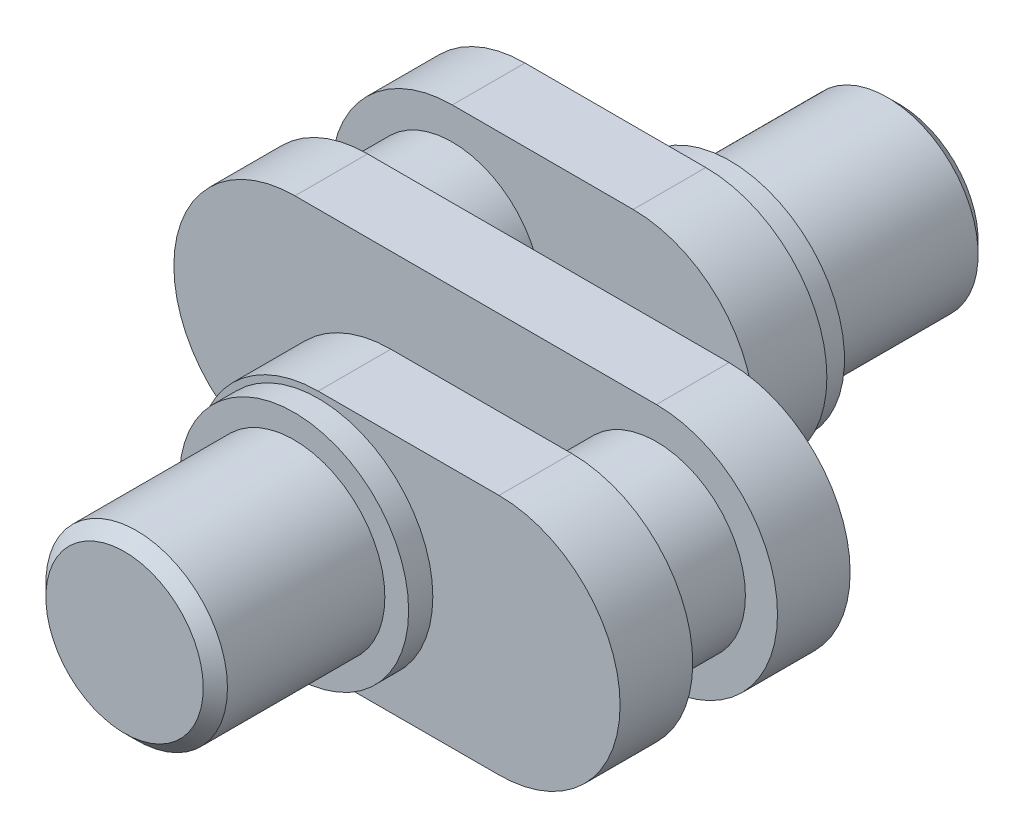
from build123d import *

# Parameters (mm, degrees)
BOSS_EXTRUDE7_DEPTH  = 3
SKETCH7_R            = 3.674588618
BOSS_EXTRUDE8_DEPTH  = 3.5
SKETCH8_R            = 3.674588618
BOSS_EXTRUDE9_DEPTH  = 3.5
SKETCH9_R            = 3.674588618
BOSS_EXTRUDE10_DEPTH = 3
SKETCH10_R           = 3.674588618
BOSS_EXTRUDE11_DEPTH = 3
SKETCH11_R           = 4.731271099
BOSS_EXTRUDE12_DEPTH = 1
SKETCH12_R           = 3.75
BOSS_EXTRUDE13_DEPTH = 7
BOSS_EXTRUDE14_START = 1
SKETCH13_R           = 4.731271099
BOSS_EXTRUDE14_DEPTH = 1
BOSS_EXTRUDE15_START = 7
SKETCH14_R           = 3.75
BOSS_EXTRUDE15_DEPTH = 7
CHAMFER1_SIZE        = 0.5


with BuildPart() as part:
    # Sketch1 → Boss-Extrude7 (new body)
    with BuildSketch(Plane.XY):
        with BuildLine():
            Line((-7.464079644, 5.007711231), (7.464079644, 5.007711231))
            ThreePointArc((7.464079644, 5.007711231), (12.46407809, 0.007713678), (7.464080538, -4.992284768))
            Line((7.464080538, -4.992284768), (-7.464079644, -4.992286102))
            ThreePointArc((-7.464079644, -4.992286102), (-12.464078311, 0.007712565), (-7.464079644, 5.007711231))
        make_face()
    extrude(amount=-BOSS_EXTRUDE7_DEPTH)

    # Sketch7 → Boss-Extrude8 (add)
    with BuildSketch(Plane(origin=(0, 0, -3), x_dir=(-1, 0, 0), z_dir=(0, 0, -1))):
        with Locations(Location((7.464079644, 0.007712565, 0), (0, 0, 180))):
            Circle(SKETCH7_R)
    extrude(amount=BOSS_EXTRUDE8_DEPTH)

    # Sketch8 → Boss-Extrude9 (add)
    with BuildSketch(Plane.XY):
        with Locations((7.464079644, 0.007712565)):
            Circle(SKETCH8_R)
    extrude(amount=BOSS_EXTRUDE9_DEPTH)

    # Sketch9 → Boss-Extrude10 (add)
    # profile 1 of 2: a face of its own
    with BuildSketch(Plane(origin=(0, 0, -6.5), x_dir=(-1, 0, 0), z_dir=(0, 0, -1))):
        with BuildLine():
            Line((7.458914982, 5.007708564), (-0.003874001, 5.003854283))
            ThreePointArc((-0.003874001, 5.003854283), (-5.003216645, -0.001949753), (0.003880454, -4.999997327))
            Line((0.003880454, -4.999997327), (7.464079644, -4.992284768))
            ThreePointArc((7.464079644, -4.992284768), (12.464077644, 0.007713232), (7.464079644, 5.007711231))
            Line((7.464079644, 5.007711231), (7.458914982, 5.007708564))
        make_face()
        with Locations(Location((7.464079644, 0.007712565, 0), (0, 0, 180))):
            Circle(SKETCH9_R, mode=Mode.SUBTRACT)
    # profile 2 of 2: a face of its own
    with BuildSketch(Plane(origin=(0, 0, -6.5), x_dir=(-1, 0, 0), z_dir=(0, 0, -1))):
        with Locations(Location((7.464079644, 0.007712565, 0), (0, 0, 180))):
            Circle(SKETCH9_R)
    extrude(amount=BOSS_EXTRUDE10_DEPTH)

    # Sketch10 → Boss-Extrude11 (add)
    # profile 1 of 2: a face of its own
    with BuildSketch(Plane.XY.offset(3.5)):
        with BuildLine():
            ThreePointArc((-0.003873651, 5.003854283), (-5.003216178, -0.00216555), (0.004312288, -4.999996973))
            Line((0.004312288, -4.999996973), (7.3891908, -4.991725236))
            ThreePointArc((7.3891908, -4.991725236), (12.463938092, -0.029732908), (7.464079644, 5.007711231))
            Line((7.464079644, 5.007711231), (7.458914981, 5.007708564))
            Line((7.458914981, 5.007708564), (-0.003873651, 5.003854283))
        make_face()
        with Locations((7.464079644, 0.007712565)):
            Circle(SKETCH10_R, mode=Mode.SUBTRACT)
    # profile 2 of 2: a face of its own
    with BuildSketch(Plane.XY.offset(3.5)):
        with Locations((7.464079644, 0.007712565)):
            Circle(SKETCH10_R)
    extrude(amount=BOSS_EXTRUDE11_DEPTH)

    # Sketch11 → Boss-Extrude12 (add)
    with BuildSketch(Plane.XY.offset(6.5)):
        with Locations((1e-09, 0.015425152)):
            Circle(SKETCH11_R)
    extrude(amount=BOSS_EXTRUDE12_DEPTH)

    # Sketch12 → Boss-Extrude13 (add)
    with BuildSketch(Plane.XY.offset(7.5)):
        with Locations((1e-09, 0.015425152)):
            Circle(SKETCH12_R)
    extrude(amount=BOSS_EXTRUDE13_DEPTH)

    # Sketch13 → Boss-Extrude14 (add)
    with BuildSketch(Plane(origin=(0, 0, -9.5), x_dir=(-1, 0, 0), z_dir=(0, 0, -1)).offset(BOSS_EXTRUDE14_START)):
        with Locations(Location((-1e-09, 0.015425152, 0), (0, 0, 180))):
            Circle(SKETCH13_R)
    extrude(amount=-BOSS_EXTRUDE14_DEPTH)

    # Sketch14 → Boss-Extrude15 (add)
    with BuildSketch(Plane(origin=(0, 0, -10.5), x_dir=(-1, 0, 0), z_dir=(0, 0, -1)).offset(BOSS_EXTRUDE15_START)):
        with Locations(Location((-1e-09, 0.015425152, 0), (0, 0, 180))):
            Circle(SKETCH14_R)
    extrude(amount=-BOSS_EXTRUDE15_DEPTH)

    # Chamfer1
    chamfer1_edges = [part.edges().sort_by_distance(p)[0] for p in [
        (-3.749999999, 0.015425152, 14.5),
        (-3.749999999, 0.015425152, -17.5),
    ]]
    chamfer(chamfer1_edges, length=CHAMFER1_SIZE)


solid = part.part
